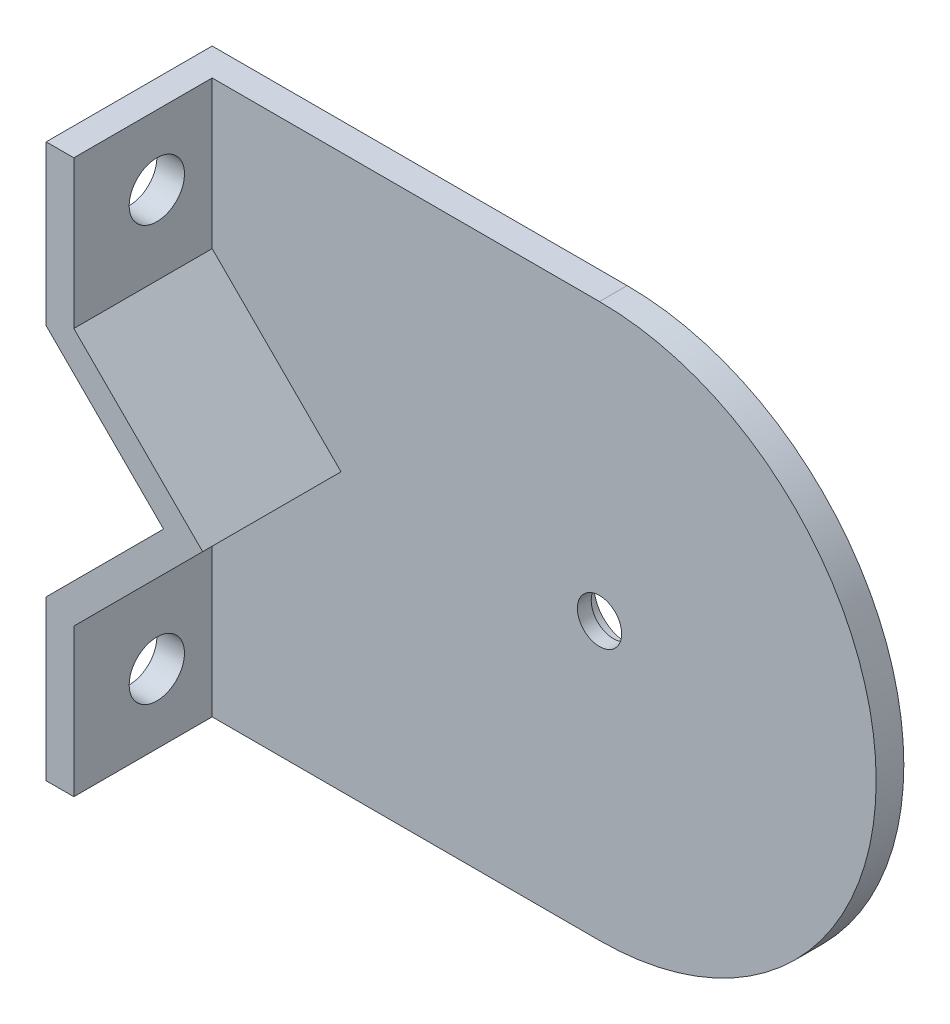
from build123d import *

# Parameters (mm, degrees)
SKETCH_1_R          = 8
EXTRUDE_1_DEPTH     = 10
EXTRUDE_2_DEPTH     = 50
CUT_EXTRUDE_1_DEPTH = 188.082869339
SKETCH_4_R          = 10
CUT_EXTRUDE_2_DEPTH = 40
SKETCH_6_R          = 12
CUT_EXTRUDE_4_DEPTH = 5


with BuildPart() as part:
    # 草图1 → 凸台-拉伸1 (new body)
    with BuildSketch(Plane.XY):
        with BuildLine():
            Line((0, 100), (-150, 100))
            Line((-150, 100), (-150, -100))
            Line((-150, -100), (0, -100))
            ThreePointArc((0, -100), (100, 0), (0, 100))
        make_face()
        Circle(SKETCH_1_R, mode=Mode.SUBTRACT)
    extrude(amount=EXTRUDE_1_DEPTH)

    # 草图2 → 凸台-拉伸2 (add)
    with BuildSketch(Plane.XY.offset(10)):
        Polygon((-150, 42.426406871), (-150, 100), (-140, 100), (-140, 46.568542495), (-93.431457505, 0), (-140, -46.568542495), (-140, -100), (-150, -100), (-150, -42.426406871), (-107.573593129, 0), align=None)
    extrude(amount=EXTRUDE_2_DEPTH)

    # 草图3 → 切除-拉伸1 (cut, through all)
    with BuildSketch(Plane.XY.offset(10)):
        Polygon((-150, -42.426406871), (-107.573593129, 0), (-150, 42.426406871), align=None)
    extrude(amount=-CUT_EXTRUDE_1_DEPTH, mode=Mode.SUBTRACT)

    # 草图4 → 切除-拉伸2 (cut)
    with BuildSketch(Plane.ZY.offset(150)):
        with Locations((30, -75)):
            Circle(SKETCH_4_R)
        with Locations((30, 75)):
            Circle(SKETCH_4_R)
    extrude(amount=-CUT_EXTRUDE_2_DEPTH, mode=Mode.SUBTRACT)

    # 草图6 → 切除-拉伸4 (cut)
    with BuildSketch(Plane(origin=(0, 0, 0), x_dir=(-1, 0, 0), z_dir=(0, 0, -1))):
        Circle(SKETCH_6_R)
    extrude(amount=-CUT_EXTRUDE_4_DEPTH, mode=Mode.SUBTRACT)


solid = part.part
